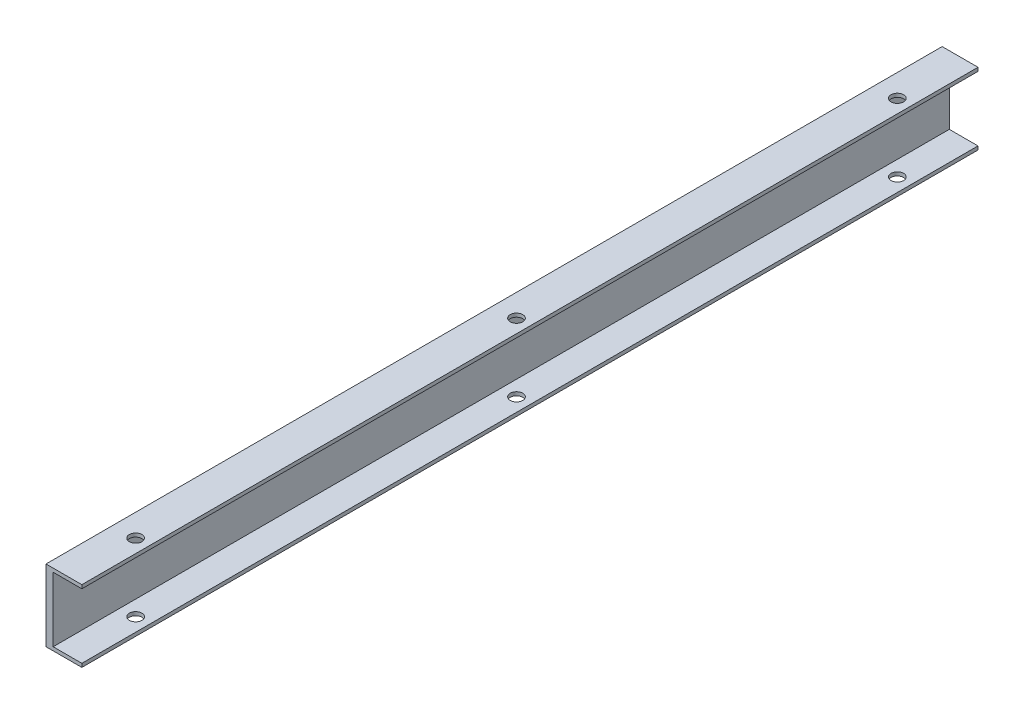
SolidWorks part; units mm, degrees
ref_plane "Front Plane" through (0, 0, 0) normal (0, 0, 1) x (1, 0, 0)
ref_plane "Top Plane" through (0, 0, 0) normal (0, 1, 0) x (1, 0, 0)
ref_plane "Right Plane" through (0, 0, 0) normal (1, 0, 0) x (0, 0, -1)
sketch "Sketch1" plane through (0, 0, 0) normal (0, 0, 1) x (1, 0, 0)
  line L0 (0, 0) -> (-40, 0)
  line L1 (-40, 0) -> (-40, 80)
  line L2 (-40, 80) -> (0, 80)
  line L3 (0, 80) -> (0, 76)
  line L4 (0, 76) -> (-32, 76)
  line L5 (-32, 76) -> (-32, 4)
  line L6 (-32, 4) -> (0, 4)
  line L7 (0, 4) -> (0, 0)
  dimension "D1" = 80
  dimension "D2" = 40
  dimension "D3" = 40
  dimension "D4" = 4
  dimension "D5" = 4
  dimension "D6" = 8
sheet metal parameters "Sheet metal 1" thickness 3 parameters "D1"=3
extrude "Extrude1" add sketch "Sketch1" along normal blind 1000
sketch "Sketch2" plane through (0, 80, 0) normal (0, 1, 0) x (1, 0, 0)
  line L0 (-40, -1000) -> (-40, 0) construction
  line L1 (0, -1000) -> (0, 0) construction
  circle A0 centre (-15, -925) radius 7
  point P4 (0, -500)
  dimension "D2" = 14
  dimension "D1" = 25
  dimension "D3" = 425
extrude "Cut-Extrude1" cut sketch "Sketch2" against normal through all
pattern_linear "LPattern1" count 3 spacing 425 along (0, 0, -1) of "Cut-Extrude1"
